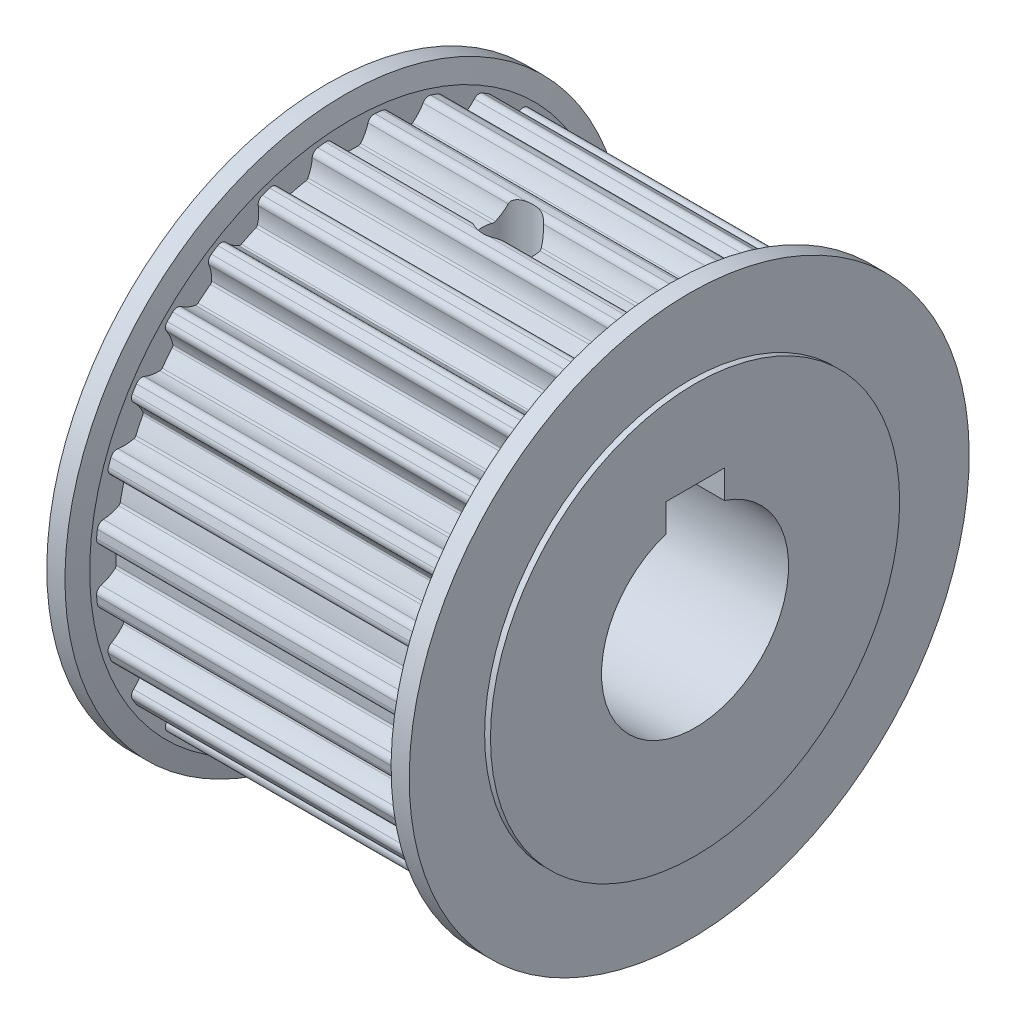
SolidWorks part; units mm, degrees
ref_plane "Front Plane" through (0, 0, 0) normal (0, 0, 1) x (1, 0, 0)
ref_plane "Top Plane" through (0, 0, 0) normal (0, 1, 0) x (1, 0, 0)
ref_plane "Right Plane" through (0, 0, 0) normal (1, 0, 0) x (0, 0, -1)
sketch "Sketch1" plane through (0, 0, 0) normal (0, 0, 1) x (1, 0, 0)
  line L0 (-13.5, 21.8) -> (-13.5, 17.5)
  line L1 (-13.5, 21.8) -> (13.5, 21.8)
  line L2 (13.5, 21.8) -> (13.5, 17.5)
  line L3 (13.5, 17.5) -> (16, 17.5)
  line L4 (16, 17.5) -> (16, 0)
  line L5 (16, 0) -> (-16, 0)
  line L6 (-13.5, 17.5) -> (-16, 17.5)
  line L7 (-16, 17.5) -> (-16, 0)
  dimension "D1" = 17.5
  dimension "D2" = 27
  dimension "D3" = 32
  dimension "D4" = 21.8
revolve "Revolve1" add sketch "Sketch1" angle 360 about L5
sketch "Sketch2" plane through (13.5, 0, 0) normal (1, 0, 0) x (0, 0, -1)
  line L2 (0, 21.8) -> (0, 20.03) construction
  arc A0 (1.625, 21.7394) -> (-1.625, 21.7394) centre (0, 0) ccw
  arc A1 (0.8048, 20.0138) -> (-0.8048, 20.0138) centre (0, 0) ccw
  circle A2 centre (0, 0) radius 21.8 construction
  circle A3 centre (0, 0) radius 22.28 construction
  circle A4 centre (0, 0) radius 21.8 construction
  arc A5 (0.8048, 20.0138) -> (1.625, 21.7394) centre (-1.6143, 22.2214) ccw
  arc A6 (-0.8048, 20.0138) -> (-1.625, 21.7394) centre (1.6143, 22.2214) cw
  dimension "D1" = 1.77
  dimension "D2" = 44.56
  dimension "D4" = 3.275
  dimension "D3" = 3.25
extrude "Cut-Extrude1" cut sketch "Sketch2" against normal through all
fillet "Fillet1" radius 0.25 2 edges at (0, 20.0138, 0.8048) (0, 20.0138, -0.8048)
fillet "Fillet2" radius 0.55 2 edges at (0, 21.7394, 1.625) (0, 21.7394, -1.625)
pattern_circular "CirPattern1" count 28 over 360 about axis through (0, 0, 0) along (1, 0, 0) of "Fillet2", "Fillet1", "Cut-Extrude1"
sketch "Sketch3" plane through (0, 0, 0) normal (0, 0, 1) x (1, 0, 0)
  line L0 (-15.5, 23.95) -> (-15.5, 17.5)
  line L1 (15.5, 23.95) -> (15.5, 17.5)
  line L2 (-15.5, 23.95) -> (-13.9475, 23.95)
  line L3 (-13.9475, 23.95) -> (-13.5, 22.28)
  line L4 (-13.5, 22.28) -> (-13.5, 17.5)
  line L5 (-13.5, 17.5) -> (-15.5, 17.5)
  line L6 (-13.5, 17.5) -> (-16, 17.5) construction
  line L8 (16, 0) -> (-16, 0) construction
  line L10 (-16, 17.5) -> (-16, -17.5) construction
  line L11 (0, 0) -> (0, 10.534) construction
  line L14 (15.5, 23.95) -> (13.9475, 23.95)
  line L15 (13.9475, 23.95) -> (13.5, 22.28)
  line L16 (13.5, 22.28) -> (13.5, 17.5)
  line L17 (13.5, 17.5) -> (15.5, 17.5)
  line L20 (16, -17.5) -> (16, 17.5) construction
  dimension "D1" = 15
  dimension "D2" = 2
  dimension "D3" = 22.28
  dimension "D4" = 23.95
revolve "Revolve3" add sketch "Sketch3" angle 360 about L8
sketch "Sketch4" [suppressed] plane through (0, 0, 0) normal (0, 0, 1) x (1, 0, 0)
  line L1 (8, 0) -> (20, 0)
  line L2 (8, 0) -> (8, 7)
  line L3 (8, 7) -> (20, 7)
  line L4 (20, 0) -> (20, 7)
  line L6 (8, -8) -> (8, 8) construction
  dimension "D1" = 16
  dimension "D2" = -4
revolve "Revolve4" [suppressed] add sketch "Sketch4" angle 360 about L1
sketch "Sketch7" [suppressed] plane through (-8, 0, 0) normal (-1, 0, 0) x (0, 0, 1)
  circle A0 centre (0, 0) radius 4
  dimension "D1" = 16
extrude "Cut-Extrude3" [suppressed] cut sketch "Sketch7" against normal through all
sketch "Sketch8" plane through (-16, 0, 0) normal (-1, 0, 0) x (0, 0, 1)
  line L0 (-2.5, 7.5993) -> (-2.5, 10)
  line L1 (-2.5, 10) -> (2.5, 10)
  line L2 (2.5, 10) -> (2.5, 7.5993)
  arc A0 (-2.5, 7.5993) -> (2.5, 7.5993) centre (0, 0) ccw
  dimension "D1" = 8
  dimension "D2" = 5
  dimension "D3" = 10
extrude "Cut-Extrude4" cut sketch "Sketch8" against normal through all
sketch "Sketch13" plane through (0, 0, 0) normal (0, 0, 1) x (1, 0, 0)
  line L0 (0, 0) -> (21.5, 0) construction
ref_plane "Plane1" through (0, 0, 0) normal (0, 0.866, -0.5) x (1, 0, 0)
sketch "Sketch24" plane through (0, 0, 0) normal (0, 0, 1) x (1, 0, 0)
  line L1 (0, 0) -> (2.15, 0)
  line L2 (0, 0) -> (0, 21.8)
  line L3 (0, 21.8) -> (2.15, 21.8)
  line L4 (2.15, 0) -> (2.15, 21.8)
  dimension "D1" = 2.15
  dimension "D2" = 21.8
revolve "Cut-Revolve8" cut sketch "Sketch24" angle 360 about L2
cosmetic thread "Cosmetic Thread7" parameters "D2"=5
sketch "Sketch25" plane through (0, 0, 0) normal (0, 0.866, -0.5) x (1, 0, 0)
  line L1 (0, 0) -> (-2.15, 0)
  line L2 (0, 0) -> (0, 21.8)
  line L3 (0, 21.8) -> (-2.15, 21.8)
  line L4 (-2.15, 0) -> (-2.15, 21.8)
  dimension "D1" = 2.15
  dimension "D2" = 21.8
revolve "Cut-Revolve9" cut sketch "Sketch25" angle 360 about L2
cosmetic thread "Cosmetic Thread6" parameters "D2"=5
sketch "Sketch9" [suppressed] plane through (-8, 0, 0) normal (-1, 0, 0) x (0, 0, 1)
  circle A0 centre (0, 0) radius 4.5
  dimension "D1" = 9
extrude "Cut-Extrude5" [suppressed] cut sketch "Sketch9" against normal blind 3
sketch "Sketch11" [suppressed] plane through (0, 0, 0) normal (0, 0, 1) x (1, 0, 0)
  line L0 (-8, 4.5) -> (-5, 4.5)
  line L1 (-8, 8) -> (-8, -8) construction
  line L2 (-5, 4.5) -> (-5, 0)
  line L3 (-5, 0) -> (-8, 0)
  line L4 (-8, 0) -> (-8, 4.5)
  line L5 (5, 0) -> (5, 4.5)
  line L6 (5, 4.5) -> (8, 4.5)
  line L7 (8, -8) -> (8, 8) construction
  line L8 (8, 4.5) -> (8, 0)
  line L9 (8, 0) -> (5, 0)
  dimension "D1" = 3
  dimension "D2" = 3
  dimension "D3" = 4.5
  dimension "D4" = 4.5
revolve "Cut-Revolve1" [suppressed] cut sketch "Sketch11" angle 360 about L3
sketch "Sketch12" [suppressed] plane through (0, 0, 0) normal (0, 0, 1) x (1, 0, 0)
  line L0 (20, 7) -> (8, 7) construction
  line L1 (13, 7) -> (11.28, 7)
  line L2 (13, 7) -> (13, 0)
  line L3 (13, 0) -> (11.28, 0)
  line L4 (11.28, 7) -> (11.28, 0)
  line L5 (20, -7) -> (20, 7) construction
  dimension "D1" = 7
  dimension "D2" = 2.15
revolve "Cut-Revolve2" cut sketch "Sketch12" angle 360 about L2
cosmetic thread "Cosmetic Thread2" [suppressed] parameters "D2"=5
sketch "Sketch14" [suppressed] plane through (0, 0, 0) normal (0, 0.866, -0.5) x (1, 0, 0)
  line L0 (20, 7) -> (8, 7) construction
  line L1 (13, 7) -> (11.28, 7)
  line L2 (13, 7) -> (13, 0)
  line L3 (13, 0) -> (11.28, 0)
  line L4 (11.28, 7) -> (11.28, 0)
  line L5 (20, -7) -> (20, 7) construction
  dimension "D1" = 7
  dimension "D2" = 2.15
revolve "Cut-Revolve3" cut sketch "Sketch14" angle 360 about L2
cosmetic thread "Cosmetic Thread1" [suppressed] parameters "D2"=5
sketch "Sketch15" [suppressed] plane through (20, 0, 0) normal (1, 0, 0) x (0, 0, -1)
  circle A0 centre (0, 0) radius 4.5
  dimension "D1" = 9
extrude "Cut-Extrude6" [suppressed] cut sketch "Sketch15" against normal blind 3
sketch "Sketch22" [suppressed] plane through (0, 0, 0) normal (0, 0, 1) x (1, 0, 0)
  line L0 (-1000, 0) -> (49000, 0) construction
  line L1 (-5.5, 8) -> (-10.5, 8)
  line L2 (-5.5, 8) -> (-5.5, 12.95)
  line L3 (-5.5, 12.95) -> (-10.5, 12.95)
  line L4 (-10.5, 8) -> (-10.5, 12.95)
  dimension "D1" = 13.5
  dimension "D2" = 5
  dimension "D3" = 17.5
  dimension "D4" = 23.95
revolve "Cut-Revolve6" [suppressed] cut sketch "Sketch22" angle 360 about L0
sketch "Sketch23" [suppressed] plane through (0, 0, 0) normal (0, 0, 1) x (1, 0, 0)
  line L0 (-1000, 0) -> (49000, 0) construction
  line L1 (10.5, 8) -> (5.5, 8)
  line L2 (10.5, 8) -> (10.5, 12.95)
  line L3 (10.5, 12.95) -> (5.5, 12.95)
  line L4 (5.5, 8) -> (5.5, 12.95)
  dimension "D1" = 13.5
  dimension "D2" = 5
  dimension "D3" = 23.95
  dimension "D4" = 17.5
revolve "Cut-Revolve7" [suppressed] cut sketch "Sketch23" angle 360 about L0
sketch "Sketch26" [suppressed] plane through (0, 0, 0) normal (0, 0, 1) x (1, 0, 0)
  line L0 (-1000, 0) -> (49000, 0) construction
  line L1 (25, 20) -> (-25, 20)
  line L2 (25, 20) -> (25, 12.95)
  line L3 (25, 12.95) -> (-25, 12.95)
  line L4 (-25, 20) -> (-25, 12.95)
  dimension "D1" = 20
  dimension "D2" = 23.95
  dimension "D3" = 50
  dimension "D4" = 25
revolve "Cut-Revolve10" [suppressed] cut sketch "Sketch26" angle 360 about L0
